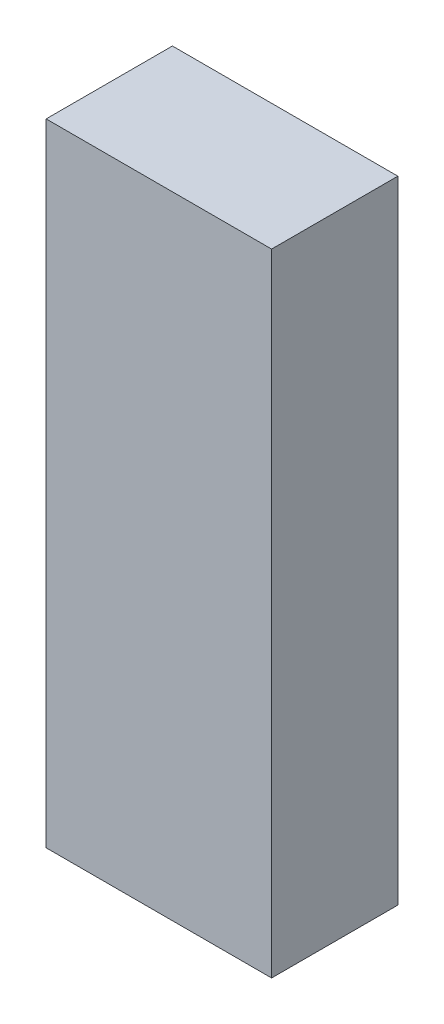
SolidWorks part; units mm, degrees
ref_plane "前视基准面" through (0, 0, 0) normal (0, 0, 1) x (1, 0, 0)
ref_plane "上视基准面" through (0, 0, 0) normal (0, 1, 0) x (1, 0, 0)
ref_plane "右视基准面" through (0, 0, 0) normal (1, 0, 0) x (0, 0, -1)
sketch "草图1" plane through (0, 0, 0) normal (0, 0, 1) x (1, 0, 0)
  line L1 (-12.5, -35) -> (12.5, -35)
  line L2 (-12.5, -35) -> (-12.5, 35)
  line L3 (-12.5, 35) -> (12.5, 35)
  line L4 (12.5, -35) -> (12.5, 35)
  line L5 (-12.5, -35) -> (12.5, 35) construction
  line L6 (-12.5, 35) -> (12.5, -35) construction
  point P0 (0, 0)
  dimension "D1" = 25
  dimension "D2" = 70
extrude "凸台-拉伸1" add sketch "草图1" along normal mid plane 14
